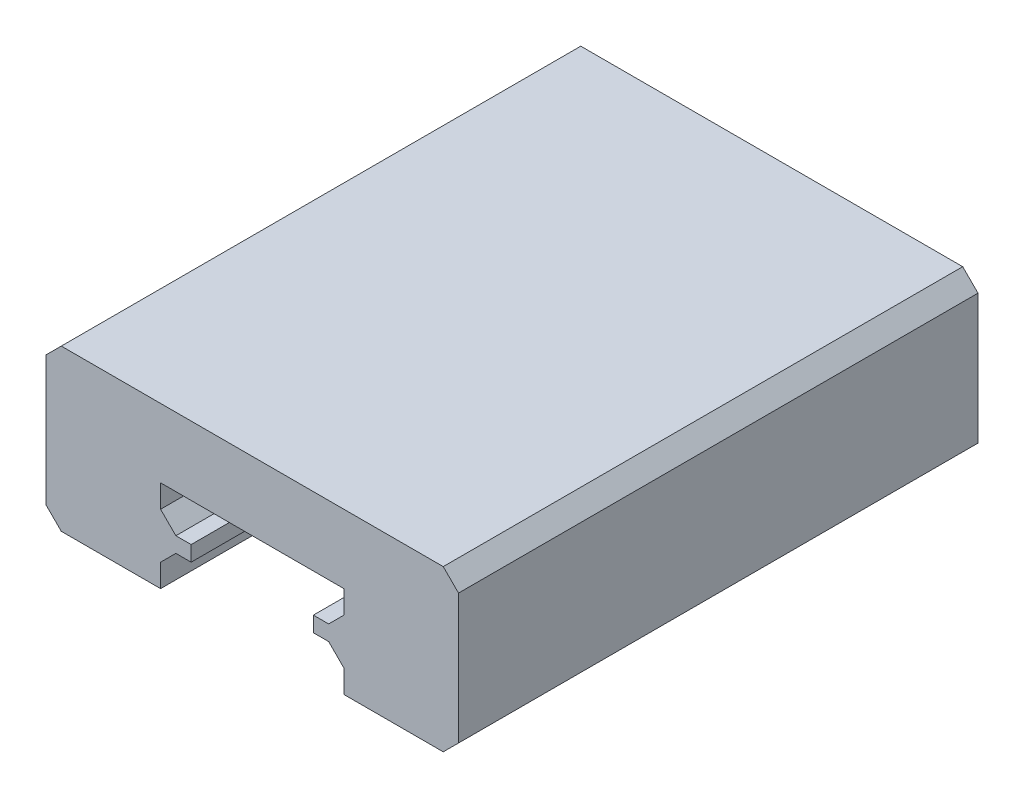
SolidWorks part; units mm, degrees
ref_plane "Front Plane" through (0, 0, 0) normal (0, 0, 1) x (1, 0, 0)
ref_plane "Top Plane" through (0, 0, 0) normal (0, 1, 0) x (1, 0, 0)
ref_plane "Right Plane" through (0, 0, 0) normal (1, 0, 0) x (0, 0, -1)
sketch "Sketch1" plane through (0, 0, 0) normal (0, 0, 1) x (1, 0, 0)
  line L0 (-13.5, -0.25) -> (13.5, -0.25) construction
  line L1 (-13.5, 5) -> (13.5, 5)
  line L2 (-13.5, 5) -> (-13.5, -5.5)
  line L3 (-13.5, -5.5) -> (-6, -5.5)
  line L4 (13.5, 5) -> (13.5, -5.5)
  line L5 (0, 5) -> (0, -5.5) construction
  line L6 (-6, 0.5) -> (-6, -1)
  line L7 (-6, 0.5) -> (6, 0.5)
  line L8 (-6, -2.5) -> (-4, -2.5) construction
  line L9 (-4, -2) -> (-4, -3)
  line L10 (-4, -2) -> (-5, -2)
  line L11 (-4, -3) -> (-5, -3)
  line L12 (-5, -2) -> (-6, -1)
  line L13 (-5, -3) -> (-6, -4)
  line L14 (6, -2.5) -> (4, -2.5) construction
  line L15 (5, -3) -> (6, -4)
  line L16 (5, -2) -> (6, -1)
  line L17 (4, -3) -> (5, -3)
  line L18 (4, -2) -> (5, -2)
  line L19 (4, -2) -> (4, -3)
  line L20 (6, 0.5) -> (6, -1)
  line L21 (6, -5.5) -> (13.5, -5.5)
  line L22 (-6, -4) -> (-6, -5.5)
  line L23 (6, -4) -> (6, -5.5)
  point P0 (0, 0)
  point P17 (-4, -2.5)
  point P31 (0, 0.5)
  dimension "D1" = 27
  dimension "D2" = 10.5
  dimension "D3" = 5
  dimension "D4" = 13.5
  dimension "D5" = 7.5
  dimension "D6" = 6
  dimension "D7" = 2
  dimension "D8" = 1
extrude "Boss-Extrude1" add sketch "Sketch1" along normal blind 34
chamfer "Chamfer1" distance 1 angle 45 4 edges at (13.5, -5.5, 17) (-13.5, -5.5, 17) (-13.5, 5, 17) (13.5, 5, 17)
